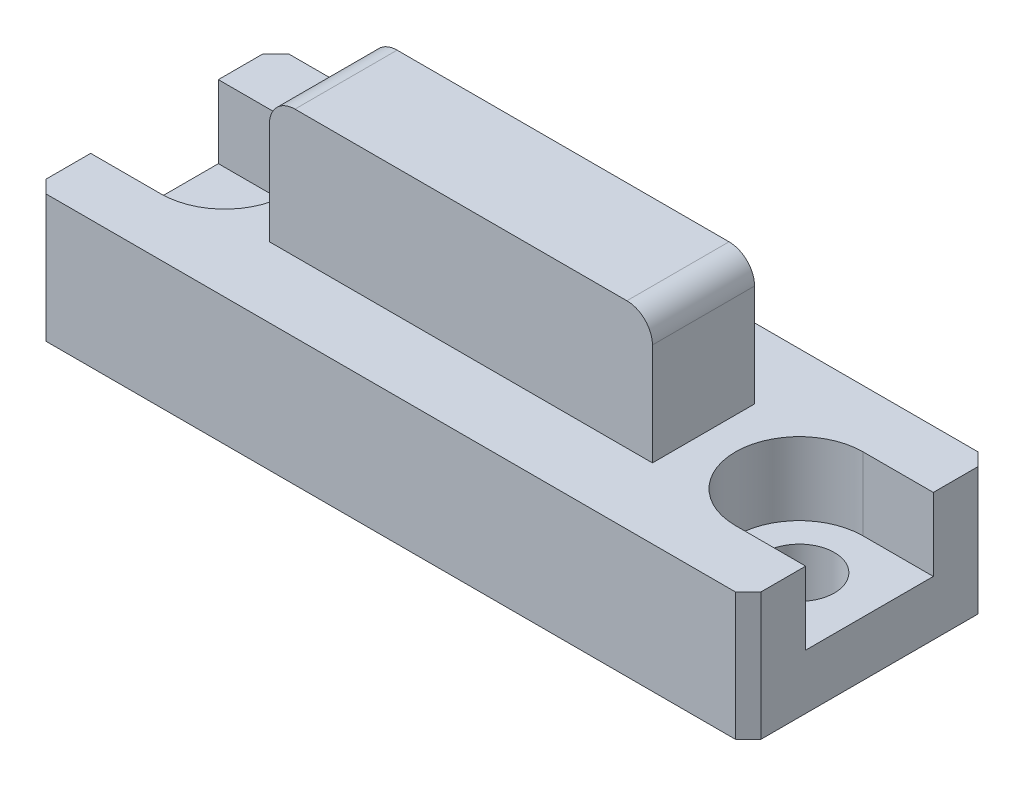
from build123d import *

# Parameters (mm, degrees)
BOSS_EXTRUDE1_DEPTH                                  = 9.5
HOLE_SIZE_PER_SOCKET_HEAD_CAP_SCREW_TYPE_D           = 5.5
HOLE_SIZE_PER_SOCKET_HEAD_CAP_SCREW_TYPE_CBORE_D     = 10
HOLE_SIZE_PER_SOCKET_HEAD_CAP_SCREW_TYPE_CBORE_DEPTH = 5.7
SKETCH4_W                                            = 5.5
SKETCH4_H                                            = 10
CUT_EXTRUDE1_DEPTH                                   = 5.7
SKETCH5_W                                            = 30
SKETCH5_H                                            = 11
CUT_EXTRUDE2_DEPTH                                   = 10
CHAMFER1_SIZE                                        = 1
FILLET1_R                                            = 2


with BuildPart() as part:
    # Sketch1 → Boss-Extrude1 (new, symmetric)
    with BuildSketch(Plane.XY):
        Polygon((28, 0), (-28, 0), (-28, 10), (-15, 10), (-15, 20), (15, 20), (15, 10), (28, 10), align=None)
    extrude(amount=BOSS_EXTRUDE1_DEPTH, both=True)

    # Hole size per socket head cap screw type 1 (through all)
    with Locations(Plane(origin=(0, 10, 0), x_dir=(-1, 0, 0), z_dir=(0, 1, 0))):
        with Locations((22.5, 0), (-22.5, 0)):
            CounterBoreHole(HOLE_SIZE_PER_SOCKET_HEAD_CAP_SCREW_TYPE_D / 2, HOLE_SIZE_PER_SOCKET_HEAD_CAP_SCREW_TYPE_CBORE_D / 2, HOLE_SIZE_PER_SOCKET_HEAD_CAP_SCREW_TYPE_CBORE_DEPTH)

    # Sketch4 → Cut-Extrude1 (cut)
    with BuildSketch(Plane(origin=(0, 10, 0), x_dir=(1, 0, 0), z_dir=(0, 1, 0))):
        with Locations((-25.25, 0)):
            Rectangle(SKETCH4_W, SKETCH4_H)
        with Locations((25.25, 0)):
            Rectangle(SKETCH4_W, SKETCH4_H)
    extrude(amount=-CUT_EXTRUDE1_DEPTH, mode=Mode.SUBTRACT)

    # Sketch5 → Cut-Extrude2 (cut)
    with BuildSketch(Plane(origin=(0, 20, 0), x_dir=(1, 0, 0), z_dir=(0, 1, 0))):
        with Locations((0, 9.5)):
            Rectangle(SKETCH5_W, SKETCH5_H)
        with Locations((0, -9.5)):
            Rectangle(SKETCH5_W, SKETCH5_H)
    extrude(amount=-CUT_EXTRUDE2_DEPTH, mode=Mode.SUBTRACT)

    # Chamfer1
    chamfer1_edges = [part.edges().sort_by_distance(p)[0] for p in [
        (-28, 5, 9.5),
        (28, 5, 9.5),
        (28, 5, -9.5),
        (-28, 5, -9.5),
    ]]
    chamfer(chamfer1_edges, length=CHAMFER1_SIZE)

    # Fillet1
    fillet1_edges = [part.edges().sort_by_distance(p)[0] for p in [
        (-15, 20, 0),
        (15, 20, 0),
    ]]
    fillet(fillet1_edges, radius=FILLET1_R)


solid = part.part
